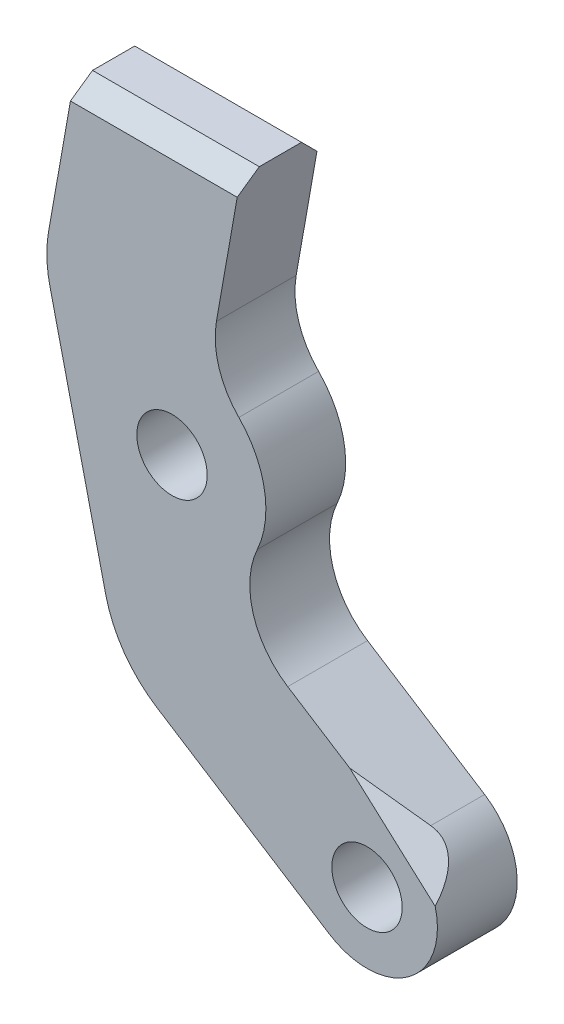
from build123d import *

# Parameters (mm, degrees)
EXTRUDE_1_DEPTH                      = 34
CHAMFER_1_SIZE                       = 8
SKETCH_2_R                           = 15
CUT_EXTRUDE_1_DEPTH                  = 275.378242911
FILLET_2_R                           = 35
FILLET_4_R                           = 50
CUT_EXTRUDE_2_REACH                  = 275.869
CUT_EXTRUDE_2_DIRECTION_2_REACH      = 275.869
CUT_EXTRUDE_2_DIRECTION_2_END_RADIUS = 30


with BuildPart() as part:
    # 草图1 → 凸台-拉伸1 (new body)
    with BuildSketch(Plane.XY):
        with BuildLine():
            Line((-125, 235), (-53.92, 235))
            Line((-53.92, 235), (-68.018431876, 155.043819614))
            ThreePointArc((-68.018431876, 155.043819614), (-43.495979684, 123.54341), (-58.429747026, 86.521672326))
            ThreePointArc((-58.429747026, 86.521672326), (-63.94761811, 82.888703808), (-69.988207372, 80.21351355))
            Line((-69.988207372, 80.21351355), (16.130569268, 25.294361725))
            ThreePointArc((16.130569268, 25.294361725), (25.294361725, -16.130569268), (-16.130569268, -25.294361725))
            Line((-16.130569268, -25.294361725), (-106.728157023, 32.480990771))
            Line((-106.728157023, 32.480990771), (-137.486072687, 164.187962972))
            Line((-137.486072687, 164.187962972), (-125, 235))
        make_face()
    extrude(amount=EXTRUDE_1_DEPTH)

    # 倒角1
    chamfer_1_edges = [part.edges().sort_by_distance(p)[0] for p in [
        (-89.46, 235, 34),
        (-89.46, 235, 0),
    ]]
    chamfer(chamfer_1_edges, length=CHAMFER_1_SIZE)

    # 草图2 → 切除-拉伸1 (cut, through all)
    with BuildSketch(Plane(origin=(0, 0, 0), x_dir=(-1, 0, 0), z_dir=(0, 0, -1))):
        with Locations((0.008418778, 0)):
            Circle(SKETCH_2_R)
        with Locations((83.120594515, 118)):
            Circle(SKETCH_2_R)
    extrude(amount=-CUT_EXTRUDE_1_DEPTH, mode=Mode.SUBTRACT)

    # 圆角2
    fillet_2_edges = [part.edges().sort_by_distance(p)[0] for p in [
        (-69.988207372, 80.21351355, 17),
        (-68.018431876, 155.043819614, 17),
    ]]
    fillet(fillet_2_edges, radius=FILLET_2_R)

    # 圆角4
    fillet_4_edges = [part.edges().sort_by_distance(p)[0] for p in [
        (-106.728157023, 32.480990771, 17),
        (-137.486072687, 164.187962972, 17),
    ]]
    fillet(fillet_4_edges, radius=FILLET_4_R)

    # 切除-拉伸2: up to this plane
    cut_extrude_2_end = Plane(origin=(-69.988207372, 80.21351355, 34), z_dir=(-0.5376856422770575, -0.8431453908366625, 0))
    # 草图4 → 切除-拉伸2 (cut, up to the surface)
    with BuildSketch(Plane(origin=(0, 0, 0), x_dir=(0, 0, -1), z_dir=(0.7431448254773932, -0.6691306063588595, 0)), mode=Mode.PRIVATE) as cut_extrude_2_sk1:
        Polygon((-34, 25), (-22, 30), (-34, 30), align=None)
    cut_extrude_2_tool1 = split(extrude(cut_extrude_2_sk1.sketch, amount=-CUT_EXTRUDE_2_REACH, mode=Mode.PRIVATE), bisect_by=cut_extrude_2_end, keep=Keep.BOTH, mode=Mode.PRIVATE)
    add(cut_extrude_2_tool1.solids().sort_by_distance((18.958701, 21.05577, 30))[0], mode=Mode.SUBTRACT)

    # 切除-拉伸2 direction 2: up to this cylinder (the profile starts inside it)
    cut_extrude_2_direction_2_end = Plane(origin=(0, 0, 30), z_dir=(0, 0, -1)) * Cylinder(CUT_EXTRUDE_2_DIRECTION_2_END_RADIUS, 612.738, mode=Mode.PRIVATE)
    # 草图4 → 切除-拉伸2 direction 2 (cut, up to the surface)
    with BuildSketch(Plane(origin=(0, 0, 0), x_dir=(0, 0, -1), z_dir=(0.7431448254773932, -0.6691306063588595, 0)), mode=Mode.PRIVATE) as cut_extrude_2_direction_2_sk1:
        Polygon((-34, 25), (-22, 30), (-34, 30), align=None)
    cut_extrude_2_direction_2_tool1 = extrude(cut_extrude_2_direction_2_sk1.sketch, amount=CUT_EXTRUDE_2_DIRECTION_2_REACH, mode=Mode.PRIVATE) & cut_extrude_2_direction_2_end
    add(cut_extrude_2_direction_2_tool1.solids().sort_by_distance((18.958701, 21.05577, 30))[0], mode=Mode.SUBTRACT)


solid = part.part
